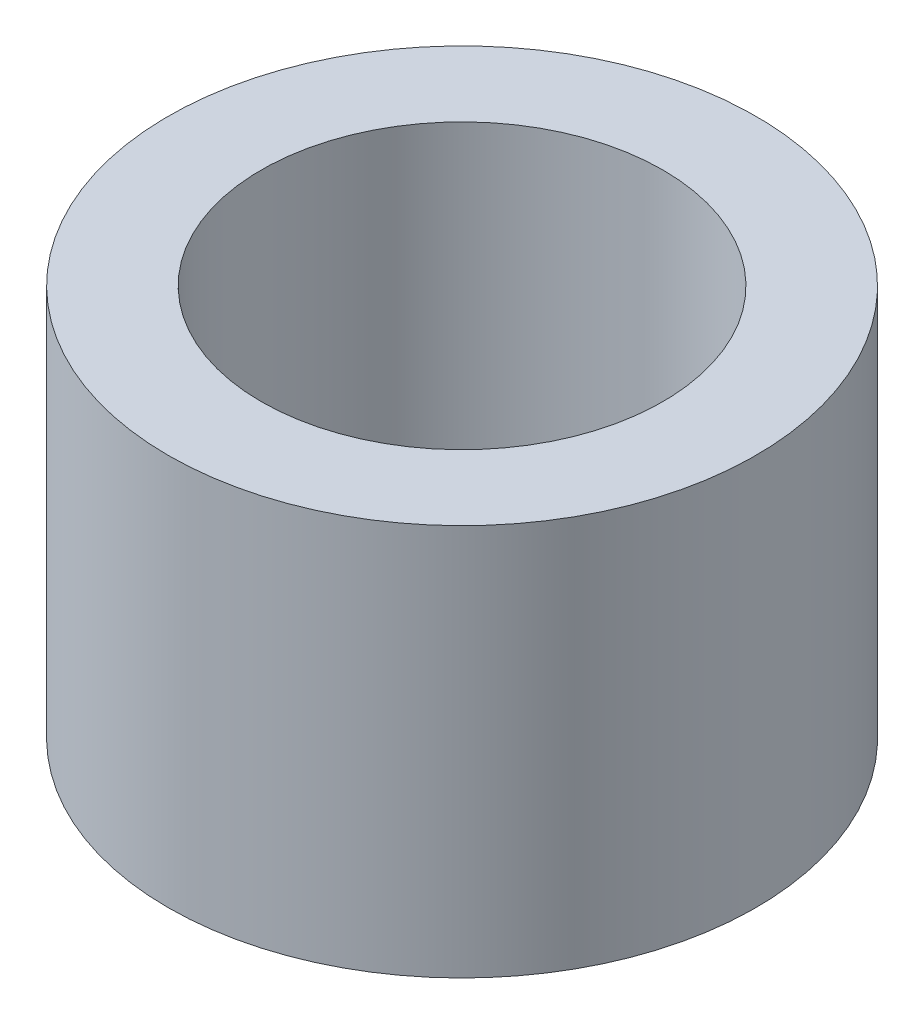
from build123d import *

# Parameters (mm, degrees)
SKETCH_1_R      = 15
SKETCH_1_R_2    = 10.25
EXTRUDE_1_DEPTH = 20


with BuildPart() as part:
    # 草图1 → 凸台-拉伸1 (new body)
    with BuildSketch(Plane(origin=(0, 0, 0), x_dir=(1, 0, 0), z_dir=(0, 1, 0))):
        with Locations(Location((0, 0, 0), (0, 0, 270))):
            Circle(SKETCH_1_R)
        with Locations(Location((0, 0, 0), (0, 0, 270))):
            Circle(SKETCH_1_R_2, mode=Mode.SUBTRACT)
    extrude(amount=EXTRUDE_1_DEPTH)


solid = part.part
